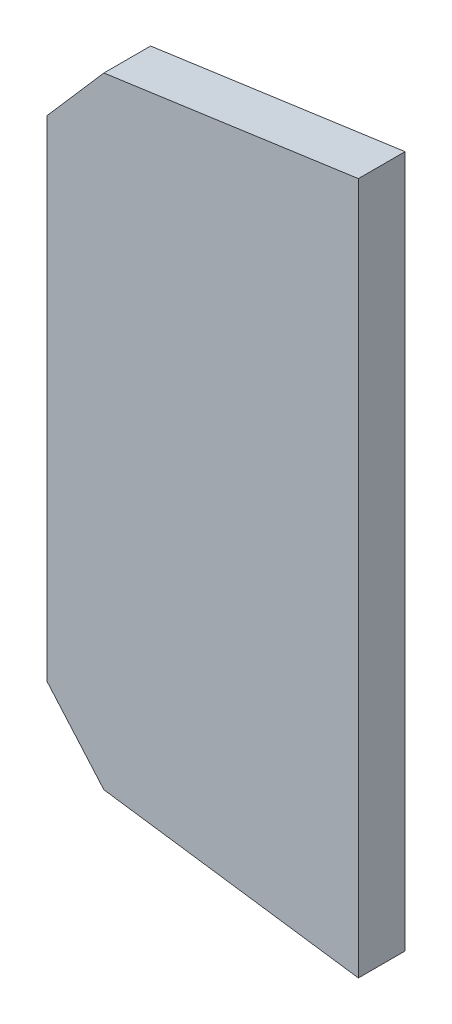
from build123d import *

# Parameters (mm, degrees)
BOSS_EXTRUDE1_DEPTH = 6


with BuildPart() as part:
    # Sketch1 → Boss-Extrude1 (new body)
    with BuildSketch(Plane.XY):
        Polygon((-4, -94.451357529), (-36.682971358, -89.858065454), (-44, -81.440786869), (-44, -18.559213131), (-36.682971358, -10.141934546), (-4, -5.548642471), align=None)
    extrude(amount=BOSS_EXTRUDE1_DEPTH)


solid = part.part
